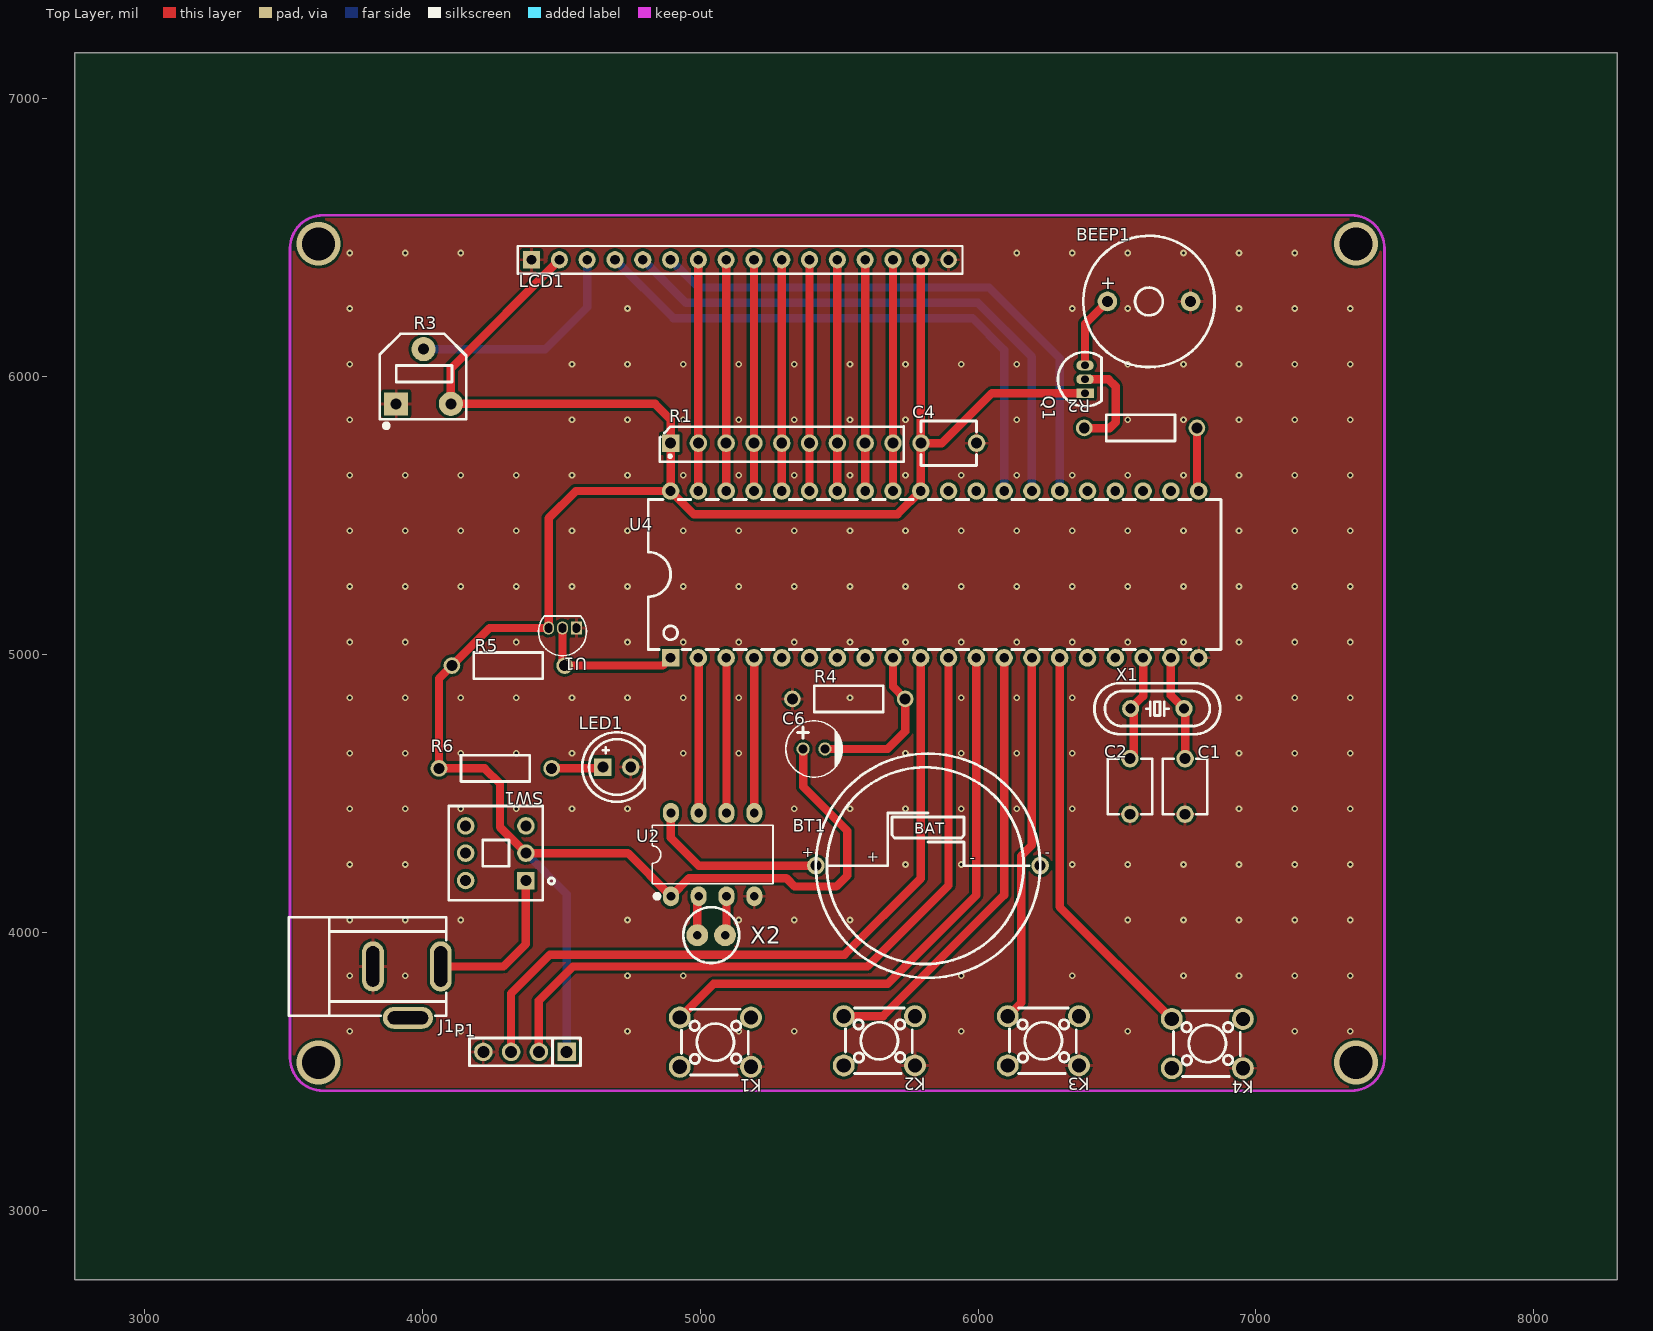
[diagram p0: Top Layer view]
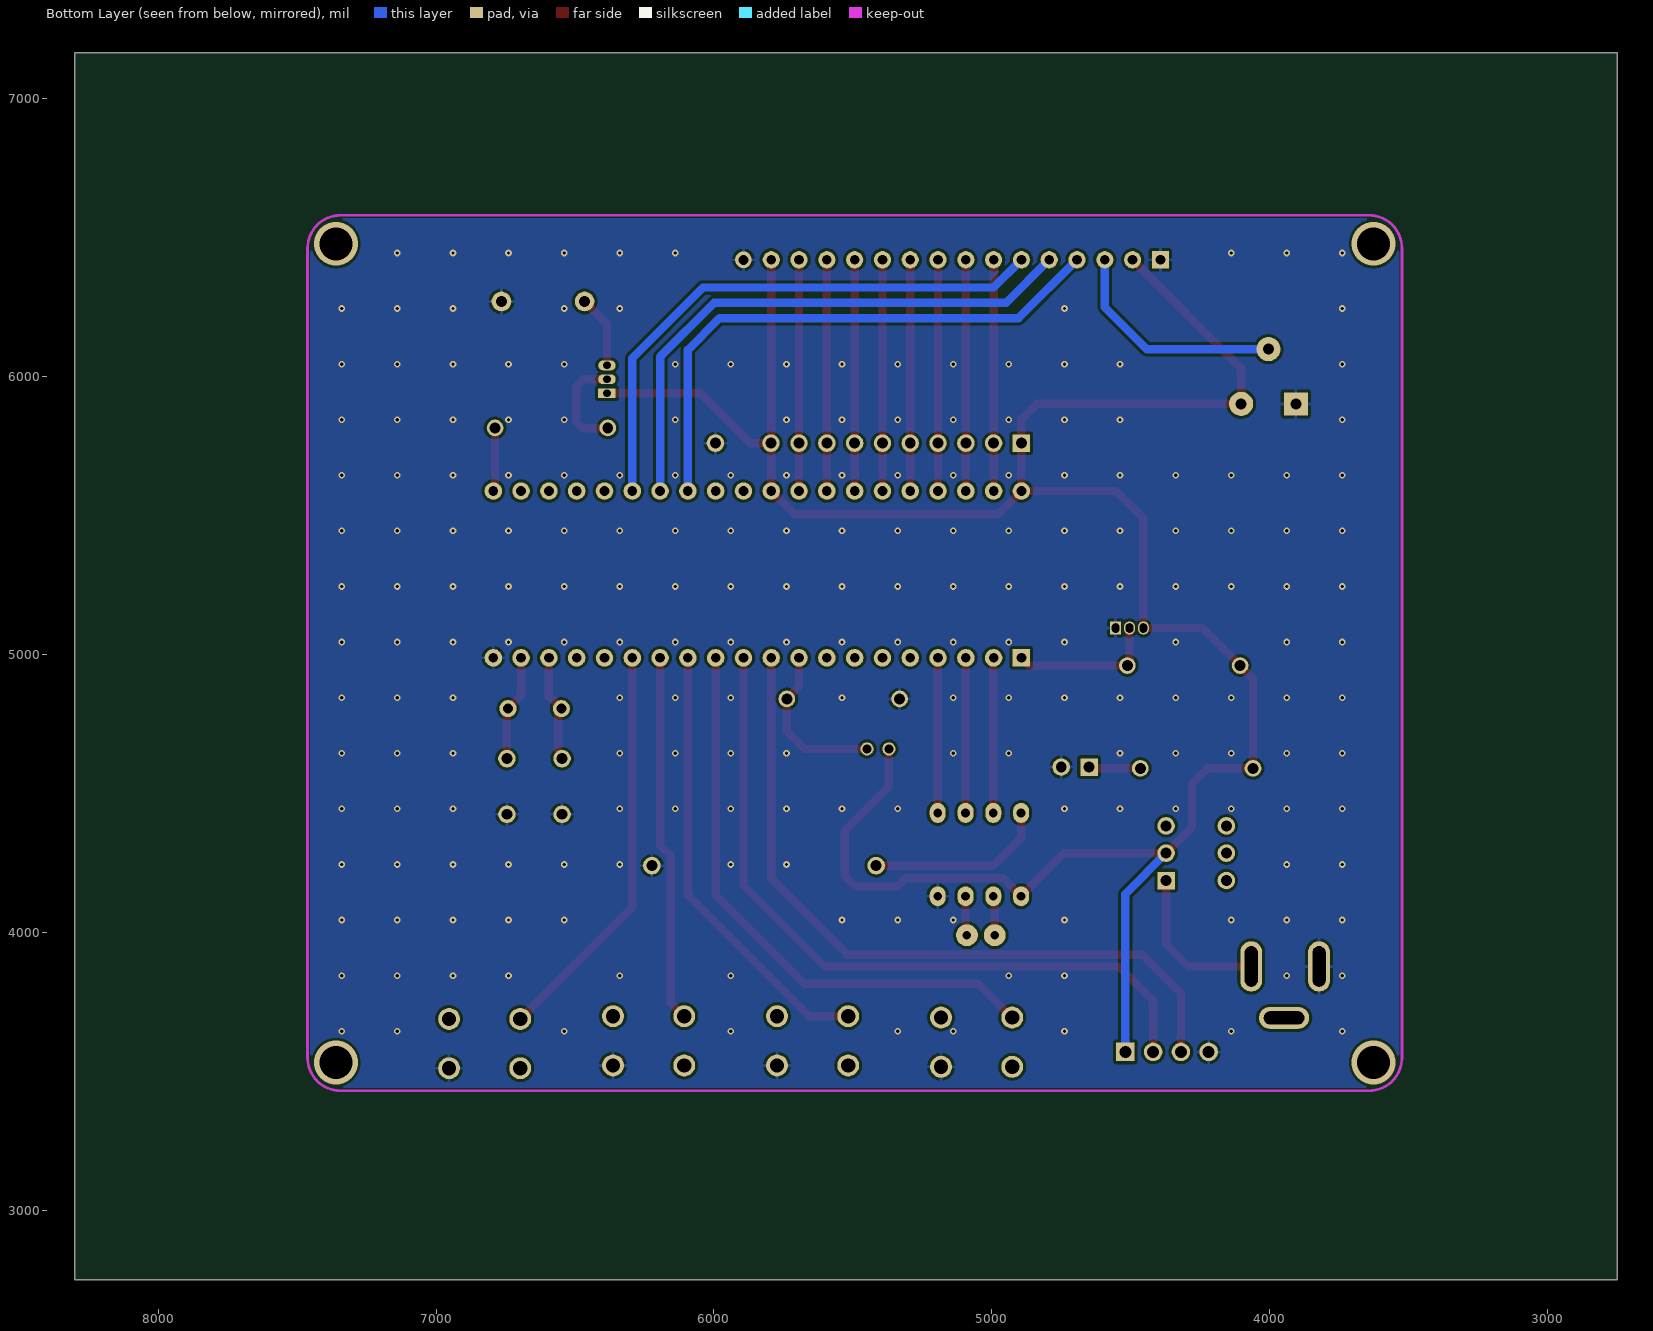
[diagram p1: Bottom Layer view, seen from below]
# Altium PCB MISC51236.pcbdoc
Units mil, origin at the board's own origin, x right, y up, seen from the top; angles counter-clockwise.
Board outline 5550 x 4415 mil, 2 copper layers (Top Layer, Bottom Layer), stack 62.206 mil thick; 27 components, 35 nets, 137 pads, 208 vias.

## Layer stack, top to bottom
Top Solder Mask Layer: solder mask 0.394, Dk 3.3
Top Layer: signal copper 1.379
Dielectric1: surface 59.449, FR4, Dk 4.5
Bottom Layer: signal copper 1.378
Bottom Solder Mask Layer: solder mask 0.394, Dk 3.3

## Board outline
8300,2750 2750,2750 2750,7165 8300,7165

## Design rules (kind name [scope] priority, off if disabled: settings)
BoardOutlineClearance copperThickness2oz_1 [All] p2 off: genericclearance=7.99 ignorepadtopadclearanceinfootprint=FALSE except(0: Arc-SplitContinuation Track-SplitContinuation SMDPad-SplitContinuation THPad-SplitContinuation Via-SplitContinuation Fill-SplitContinuation Region-SplitContinuation Poly-SplitContinuation Text-SplitContinuation Hole-SplitContinuation; 5.98: Arc-CutoutEdge SMDPad-CutoutEdge THPad-CutoutEdge Via-CutoutEdge Fill-CutoutEdge Region-CutoutEdge Text-CutoutEdge; 6.93: Hole-OutlineEdge Hole-CutoutEdge; 10: Poly-OutlineEdge Poly-CutoutEdge; 11.81: Arc-OutlineEdge Track-OutlineEdge SMDPad-OutlineEdge THPad-OutlineEdge Via-OutlineEdge Fill-OutlineEdge Region-OutlineEdge Text-OutlineEdge Track-CutoutEdge)
BoardOutlineClearance copperThickness1oz_1 [All] p4: genericclearance=4.02 ignorepadtopadclearanceinfootprint=FALSE except(0: Arc-SplitContinuation Track-SplitContinuation SMDPad-SplitContinuation THPad-SplitContinuation Via-SplitContinuation Fill-SplitContinuation Region-SplitContinuation Poly-SplitContinuation Text-SplitContinuation Hole-SplitContinuation; 6: SMDPad-CutoutEdge THPad-CutoutEdge Via-CutoutEdge Fill-CutoutEdge Region-CutoutEdge Text-CutoutEdge; 6.93: Hole-OutlineEdge Hole-CutoutEdge; 10: Poly-OutlineEdge Poly-CutoutEdge; 11.8: Arc-OutlineEdge Track-OutlineEdge SMDPad-OutlineEdge THPad-OutlineEdge Via-OutlineEdge Fill-OutlineEdge Region-OutlineEdge Text-OutlineEdge; 11.81: Arc-CutoutEdge Track-CutoutEdge)
Clearance copperThickness2oz [All] p1 off: gap=7.99 ignorepadtopadclearanceinfootprint=FALSE except(5.98: SMDPad-Track SMDPad-SMDPad THPad-Track SMDPad-THPad THPad-THPad Track-Via SMDPad-Via THPad-Via Via-Via Fill-Track Region-Track Fill-SMDPad Region-SMDPad Fill-THPad Region-THPad Fill-Via Region-Via Fill-Fill Fill-Region Region-Region Arc-Track Arc-SMDPad Arc-THPad Arc-Via Fill-Arc Region-Arc Arc-Arc Text-Track SMDPad-Text Text-THPad Text-Via Fill-Text Region-Text Arc-Text Text-Text; 6.93: Hole-Track Hole-SMDPad Hole-THPad Hole-Via Fill-Hole Region-Hole Hole-Arc Hole-Text; 10: Poly-Track Poly-SMDPad Poly-THPad Poly-Via Poly-Fill Poly-Region Poly-Poly Poly-Arc Poly-Text Poly-Hole)
Clearance copperThickness1oz [All] p3: gap=4.02 ignorepadtopadclearanceinfootprint=FALSE except(5.98: SMDPad-Track SMDPad-SMDPad THPad-Track SMDPad-THPad THPad-THPad Track-Via SMDPad-Via THPad-Via Via-Via Fill-Track Region-Track Fill-SMDPad Region-SMDPad Fill-THPad Region-THPad Fill-Via Region-Via Fill-Fill Fill-Region Region-Region; 6: Arc-Track Arc-SMDPad Arc-THPad Arc-Via Fill-Arc Region-Arc Arc-Arc Text-Track SMDPad-Text Text-THPad Text-Via Fill-Text Region-Text Arc-Text Text-Text; 6.93: Hole-Track Hole-SMDPad Hole-THPad Hole-Via Fill-Hole Region-Hole Hole-Arc Hole-Text; 10: Poly-Track Poly-SMDPad Poly-THPad Poly-Via Poly-Fill Poly-Region Poly-Poly Poly-Arc Poly-Text Poly-Hole)
DiffPairsRouting differentialPair [All] p1: maxlimit=6 minlimit=6 mostfreqgap=6 toplayer_minwidth=5 toplayer_prefwidth=10 toplayer_maxwidth=100 toplayer_mingap=6 toplayer_prefgap=6 toplayer_maxgap=6 bottomlayer_minwidth=5 bottomlayer_prefwidth=10 bottomlayer_maxwidth=100 bottomlayer_mingap=6 bottomlayer_prefgap=6 bottomlayer_maxgap=6 maxuncoupledlength=179724.41
HoleToHoleClearance otherClearance [All] p1: gap=11.81 allowstackedmicrovias=TRUE
Length netLength [All] p1: minlimit=0 maxlimit=0
MatchedLengths netLengthTolerance [All] p1: tolerance=1000
PasteMaskExpansion pasteMaskExpansion [All] p1: expansion=0
PlaneConnect innerPlane [All] p1: planeconnectstyle=Relief reliefexpansion=20 reliefentries=4 reliefconductorwidth=10 reliefairgap=10
PolygonConnect copperRegion [All] p1: connectstyle=Relief reliefconductorwidth=10 reliefentries=4 polygonreliefangle="90 Angle" airgapwidth=10 via.connectstyle=Relief via.reliefconductorwidth=10 via.reliefentries=4 via.polygonreliefangle="90 Angle" via.airgapwidth=10
RoutingVias viaSize [All] p1: holewidth=12.01 width=24.02 viastyle="Through Hole" minholewidth=11.81 minwidth=19.68 maxholewidth=248.03 maxwidth=393.7
SolderMaskExpansion solderMaskExpansion [IsVia] p1: expansion=-1000 istentingtop=TRUE
SolderMaskExpansion solderMaskExpansion [All] p2: expansion=2 istentingtop=FALSE
Width copperThickness2oz_2 [All] p1 off: maxlimit=100 minlimit=8 preferedwidth=10
Width copperThickness1oz_2 [All] p2: maxlimit=100 minlimit=5 preferedwidth=10

## Components (designator, comment, footprint, x,y, rotation, side; value= is the part's Value field where it differs from the comment)
BEEP1 "" BUZ-TH_BD12.0-P7.60-D0.6-FD 6615,6270 r0 top
BT1 "Battery" BAT-TH_CR2032 5820,4240 r0 top
C1 "30pF" CAP-TH_L5.0-W4.0-P5.00-D1.0 6745,4525 r90 top
C2 "30pF" CAP-TH_L5.0-W4.0-P5.00-D1.0 6546.5,4525 r90 top
C4 "0.1uF" CAP-TH_L5.0-W4.0-P5.00-D1.0 5895,5760 r0 top
C6 "10uF" CAP-TH_BD5.0-P2.00-D0.6-FD 5410,4660 r0 top
J1 "" DC-005_2.5 3940,3865 r180 top
K1 "" KEY-TH_4P-L6.0-W6.0-P4.50-LS6.50 5055,3605 r180 top
K2 "" KEY-TH_4P-L6.0-W6.0-P4.50-LS6.50 5645,3610 r180 top
K3 "" KEY-TH_4P-L6.0-W6.0-P4.50-LS6.50 6235,3610 r180 top
K4 "" KEY-TH_4P-L6.0-W6.0-P4.50-LS6.50 6825,3600 r180 top
LCD1 "1602" HDR-M-2.54_1X16 5143.88,6420 r0 top
LED1 "" LED-TH_5mm 4700.63,4595 r0 top
P1 "" HDR-TH_4P-P2.54-V-M 4370,3570 r180 top
Q1 "8550" S8550P_TO-92 6385,5990 r90 top
R1 "" SIP-9_L22.3-W3.2-P2.54_KA2284-SIP-9 5293.88,5760 r0 top
R2 "1K" Res_1/4W 6585,5815 r0 top
R3 "103" RES-ADJ-SMD_RM065-V1 4005,6000 r0 top
R4 "10K" Res_1/4W 5535,4840 r0 top
R5 "4.7K" Res_1/4W 4310,4960 r180 top
R6 "1K" Res_1/4W 4263.44,4590 r0 top
SW1 "SWT" SW-TH_6P-L8.5-W8.5-P2.50-LS5.5-BL-2 4265,4285 r90 top
U1 "DS18B20" TO-92-3_L4.5-W3.5-P1.27-L 4505,5095 r180 top
U2 "DS1302" DIP-8_L10.9-W6.4-P2.54-LS7.6-BL 5045,4280 r0 top
U4 "STC89C52RC-40I-PDIP40" DIP-40_L52.0-W13.7-P2.54-LS15.2-BL 5843.88,5287.97 r0 top
X1 "12M" HC-49S_L11.5-W4.7-P4.88 6645,4805 r0 top
X2 "32.768kHz" XTAL2 5090,3990 r180 top

## Footprints (in the part's own frame and the unit in brackets; to place one, negate y for a bottom-side part, rotate by r counter-clockwise, add the part's x,y. Pads: shape width x height; smd on the part's side, far side on the other; paste and mask are expansions set on the pad)
BAT-TH_CR2032 [mm]
  round 1.6 hole 1: 1(-10.25,0) 2(10.25,0)
  silkscreen extent -10.25,-10.25 10.25,10.25
BUZ-TH_BD12.0-P7.60-D0.6-FD [mm]
  round 1.8 hole 1: 1(-3.8,0) 2(3.8,0)
  silkscreen extent -6,-6 6,6
CAP-TH_BD5.0-P2.00-D0.6-FD [mm]
  round 1.201 hole 0.801: 1(-1,0) 2(1,0)
  silkscreen extent -2.58,-2.57 2.59,2.57
CAP-TH_L5.0-W4.0-P5.00-D1.0 [mm]
  round 1.6 hole 1: 1(-2.54,0) 2(2.54,0)
  silkscreen extent -2.54,-2.03 2.54,2.03
DC-005_2.5 [mm]
  oval 2x4.6 hole 1.2 slot 3.7 at 90 deg paste+0 mask+0.051: 1(-3.227,-0.318) 2(2.973,-0.318)
  oval 4.6x2 hole 1.2 slot 3.7 at 0 deg paste+0 mask+0.051: 3(-0.227,4.382)
  silkscreen extent -3.73,-4.82 10.67,4.18
DIP-8_L10.9-W6.4-P2.54-LS7.6-BL [mm]
  oval 1.462x1.828 hole 0.8: 1(-3.81,-3.81) 2(-1.27,-3.81) 3(1.27,-3.81) 4(3.81,-3.81) 5(3.81,3.81) 6(1.27,3.81) 7(-1.27,3.81) 8(-3.81,3.81)
  silkscreen extent -5.53,-4.01 5.53,2.67
DIP-40_L52.0-W13.7-P2.54-LS15.2-BL [mil]
  rect 63x63 hole 35: 1(-950,-300)
  round 63 hole 35: 2(-850,-300) 3(-750,-300) 4(-650,-300) 5(-550,-300) 6(-450,-300) 7(-350,-300) 8(-250,-300) 9(-150,-300) 10(-50,-300) 11(50,-300) 12(150,-300) 13(250,-300) 14(350,-300) 15(450,-300) 16(550,-300) 17(650,-300) 18(750,-300) 19(850,-300) 20(950,-300) 21(950,300) 22(850,300) 23(750,300) 24(650,300) 25(550,300) 26(450,300) 27(350,300) 28(250,300) 29(150,300) 30(50,300) 31(-50,300) 32(-150,300) 33(-250,300) 34(-350,300) 35(-450,300) 36(-550,300) 37(-650,300) 38(-750,300) 39(-850,300) 40(-950,300)
  silkscreen extent -1030,-270 1030,270
HC-49S_L11.5-W4.7-P4.88 [mm]
  round 1.56 hole 0.9: 1(-2.44,0) 2(2.44,0)
  silkscreen extent -5.75,-2.33 5.75,2.33
HDR-M-2.54_1X16 [mil]
  rect 62x62 hole 35: 1(-750,0)
  round 62 hole 35: 2(-650,0) 3(-550,0) 4(-450,0) 5(-350,0) 6(-250,0) 7(-150,0) 8(-50,0) 9(50,0) 10(150,0) 11(250,0) 12(350,0) 13(450,0) 14(550,0) 15(650,0)
  round 60 hole 36: 16(750,0)
  silkscreen extent -800,-50 800,50
HDR-TH_4P-P2.54-V-M [mm]
  rect 1.7x1.7 hole 1.1: 1(-3.81,0)
  round 1.7 hole 1.1: 2(-1.27,0) 3(1.27,0) 4(3.81,0)
  silkscreen extent -5.08,-1.27 5.08,1.27
KEY-TH_4P-L6.0-W6.0-P4.50-LS6.50 [mm]
  round 2 hole 1.3: 1(-3.25,2.25) 2(3.25,2.25) 3(-3.25,-2.25) 4(3.25,-2.25)
  silkscreen extent -3,-3 3.1,3
LED-TH_5mm [mm]
  rect 1.6x1.6 hole 1 paste+0 mask+0.051: 1(-1.27,0)
  round 1.6 hole 1 paste+0 mask+0.051: 2(1.27,0)
  silkscreen extent -3.17,-3.17 2.54,3.17
RES-ADJ-SMD_RM065-V1 [mm]
  rect 2.2x2.1 hole 1 paste+0 mask+0.05: 1(-2.5,-2.5)
  round 2.2 hole 1 paste+0 mask+0.05: 2(0,2.5) 3(2.5,-2.5)
  silkscreen extent -4,-4.7 3.9,3.9
Res_1/4W [mil]
  round 60 hole 39.37 paste+0 mask+2: 1(-202.76,0) 2(202.76,0)
  silkscreen extent -124,-47 124,47
S8550P_TO-92 [mm]
  rect 0.9x1.6 hole 0.7 paste+0 mask+0.051: 1(-1.27,0)
  oval 0.9x1.6 hole 0.7 paste+0 mask+0.051: 2(0,0) 3(1.27,0)
  silkscreen extent -2.48,-1.5 2.48,2.48
SIP-9_L22.3-W3.2-P2.54_KA2284-SIP-9 [mm]
  rect 1.6x1.6 hole 1: 1(-10.16,0)
  round 1.6 hole 1: 2(-7.62,0) 3(-5.08,0) 4(-2.54,0) 5(0,0) 6(2.54,0) 7(5.08,0) 8(7.62,0) 9(10.16,0)
  silkscreen extent -11.15,-1.69 11.15,1.52
SW-TH_6P-L8.5-W8.5-P2.50-LS5.5-BL-2 [mm]
  rect 1.6x1.6 hole 1: 1(-2.5,-2.75)
  round 1.6 hole 1: 2(0,-2.75) 3(2.5,-2.75) 4(2.5,2.75) 5(0,2.75) 6(-2.5,2.75)
  silkscreen extent -4.3,-5.36 4.3,4.3
TO-92-3_L4.5-W3.5-P1.27-L [mm]
  rect 1x1.2 hole 0.7 slot 0.85 at 90 deg: 1(-1.27,0)
  oval 1x1.2 hole 0.7 slot 0.85 at 90 deg: 2(0,0) 3(1.27,0)
  silkscreen extent -2.19,-1.1 2.19,2.52
XTAL2 [mm]
  round 2 hole 0.762: 1(0,0) 2(2.54,0)
  silkscreen extent -1.29,-2.55 3.83,2.55

## Via types
v1: diameter 24.02, hole 12, Top Layer to Bottom Layer, 204 vias
v2: diameter 157.48, hole 118.1, Top Layer to Bottom Layer, 4 vias

## Nets (pads, with @x,y where several pads share a name; then routed paths per layer and width w, separated by ;. In a path a pad name is that pad's centre, name@x,y a point inside that pad or via, vN(x,y) a via of type N, cw(c..) or ccw(c..) an arc to the next point about the centre after c; other vN are vias at no path point)
$2N34: J1.1 SW1.1 | length 568
  Top Layer w30: J1.1 4292.52,3877.51 4373.27,3958.27 SW1.1
$2N37: BEEP1.1 Q1.3 | length 263.3
  Top Layer w30: Q1.3 6385,6189.6 BEEP1.1
$2N47: U2.2 X2.2 | length 142.1
  Top Layer w30: X2.2 4990,4125 U2.2
$2N48: U2.3 X2.1 | length 142.1
  Top Layer w30: X2.1 5095,3995 U2.3
$2N51: BT1.1 U2.8 | length 652.9
  Top Layer w30: U2.8 4895,4340 4995,4240 BT1.1
$2N72: C6.2 R4.2 U4.9 | length 597.8
  Top Layer w30: C6.2 5675,4660 5737.76,4722.76 R4.2 5693.88,4883.88 U4.9
$2N199: LCD1.3 R3.2 | length 822.3
  Bottom Layer w30: R3.2 4443.43,6098.43 4593.88,6248.88 LCD1.3
$2N200: Q1.2 R2.1 | length 372.4
  Top Layer w30: R2.1 6383.45,5813.79 6473.79,5813.79 6495,5835 6495,5965 6470,5990 Q1.2
$2N202: LED1.1 R6.2 | length 186.5
  Top Layer w30: R6.2 4645.63,4590 LED1.1
BEEP: R2.2 U4.21 | length 229.6
  Top Layer w30: R2.2 6787.76,5594.09 U4.21
D0: LCD1.7 R1.2 U4.39 | length 832
  Top Layer w30: U4.39 R1.2 LCD1.7
D1: LCD1.8 R1.3 U4.38 | length 832
  Top Layer w30: U4.38 R1.3 LCD1.8
D2: LCD1.9 R1.4 U4.37 | length 832
  Top Layer w30: U4.37 R1.4 LCD1.9
D3: LCD1.10 R1.5 U4.36 | length 832
  Top Layer w30: U4.36 R1.5 LCD1.10
D4: LCD1.11 R1.6 U4.35 | length 832
  Top Layer w30: U4.35 R1.6 LCD1.11
D5: LCD1.12 R1.7 U4.34 | length 832
  Top Layer w30: U4.34 R1.7 LCD1.12
D6: LCD1.13 R1.8 U4.33 | length 832
  Top Layer w30: U4.33 R1.8 LCD1.13
D7: LCD1.14 R1.9 U4.32 | length 832
  Top Layer w30: U4.32 R1.9 LCD1.14
DQ: R5.1 U1.2 U4.1 | length 530.9
  Top Layer w30: U1.2 4505,4967.76 R5.1 4865.91,4960 U4.1
EN: LCD1.6 U4.26 | length 2024.7
  Bottom Layer w30: LCD1.6 4993.88,6320 6040,6320 6293.88,6066.12 U4.26
GND: BEEP1.2 BT1.2 C1.1 C2.1 C4.2 J1.2 K1.1 K2.1 K3.1 K4.1 LCD1.1 LCD1.16 LED1.2 P1.4 R3.1 R4.1 U1.1 U2.4 U4.20
  other v1: 3739.1,3644.49 4139.1,3644.49 4739.1,3644.49 5139.1,3644.49 5339.1,3644.49 5939.1,3644.49 6539.1,3644.49 7139.1,3644.49 7339.1,3644.49 3739.1,3844.49 3939.1,3844.49 4739.1,3844.49 4939.1,3844.49 5939.1,3844.49 6339.1,3844.49 6739.1,3844.49 6939.1,3844.49 7139.1,3844.49 7339.1,3844.49 3739.1,4044.49 3939.1,4044.49 4139.1,4044.49 4739.1,4044.49 5139.1,4044.49 5339.1,4044.49 5539.1,4044.49 6539.1,4044.49 6739.1,4044.49 6939.1,4044.49 7139.1,4044.49 7339.1,4044.49 3739.1,4244.49 3939.1,4244.49 5739.1,4244.49 5939.1,4244.49 6339.1,4244.49 6539.1,4244.49 6739.1,4244.49 6939.1,4244.49 7139.1,4244.49 7339.1,4244.49 3739.1,4444.49 3939.1,4444.49 4139.1,4444.49 4339.1,4444.49 4539.1,4444.49 4739.1,4444.49 5339.1,4444.49 5539.1,4444.49 5739.1,4444.49 5939.1,4444.49 6139.1,4444.49 6339.1,4444.49 6939.1,4444.49 7139.1,4444.49 7339.1,4444.49 3739.1,4644.49 3939.1,4644.49 4139.1,4644.49 4339.1,4644.49 4539.1,4644.49 4939.1,4644.49 5139.1,4644.49 5739.1,4644.49 5939.1,4644.49 6139.1,4644.49 6339.1,4644.49 6939.1,4644.49 7139.1,4644.49 7339.1,4644.49 3739.1,4844.49 3939.1,4844.49 4139.1,4844.49 4339.1,4844.49 4539.1,4844.49 4739.1,4844.49 4939.1,4844.49 5139.1,4844.49 5539.1,4844.49 5939.1,4844.49 6139.1,4844.49 6339.1,4844.49 6939.1,4844.49 7139.1,4844.49 7339.1,4844.49 3739.1,5044.49 3939.1,5044.49 4339.1,5044.49 4739.1,5044.49 4939.1,5044.49 5139.1,5044.49 5339.1,5044.49 5539.1,5044.49 5739.1,5044.49 5939.1,5044.49 6139.1,5044.49 6339.1,5044.49 6539.1,5044.49 6739.1,5044.49 6939.1,5044.49 7139.1,5044.49 7339.1,5044.49 3739.1,5244.49 3939.1,5244.49 4139.1,5244.49 4339.1,5244.49 4539.1,5244.49 4739.1,5244.49 4939.1,5244.49 5139.1,5244.49 5339.1,5244.49 5539.1,5244.49 5739.1,5244.49 5939.1,5244.49 6139.1,5244.49 6339.1,5244.49 6539.1,5244.49 6739.1,5244.49 6939.1,5244.49 7139.1,5244.49 7339.1,5244.49 3739.1,5444.49 3939.1,5444.49 4139.1,5444.49 4339.1,5444.49 4539.1,5444.49 4739.1,5444.49 4939.1,5444.49 5139.1,5444.49 5339.1,5444.49 5539.1,5444.49 5739.1,5444.49 5939.1,5444.49 6139.1,5444.49 6339.1,5444.49 6539.1,5444.49 6739.1,5444.49 6939.1,5444.49 7139.1,5444.49 7339.1,5444.49 3739.1,5644.49 3939.1,5644.49 4139.1,5644.49 4339.1,5644.49 4539.1,5644.49 4739.1,5644.49 4939.1,5644.49 5139.1,5644.49 5339.1,5644.49 5539.1,5644.49 5739.1,5644.49 5939.1,5644.49 6139.1,5644.49 6339.1,5644.49 6539.1,5644.49 6739.1,5644.49 6939.1,5644.49 7139.1,5644.49 7339.1,5644.49 3739.1,5844.49 4539.1,5844.49 4739.1,5844.49 4939.1,5844.49 5139.1,5844.49 5339.1,5844.49 5539.1,5844.49 5739.1,5844.49 6139.1,5844.49 6539.1,5844.49 6739.1,5844.49 6939.1,5844.49 7139.1,5844.49 7339.1,5844.49 3739.1,6044.49 4539.1,6044.49 4739.1,6044.49 4939.1,6044.49 5139.1,6044.49 5339.1,6044.49 5539.1,6044.49 5739.1,6044.49 5939.1,6044.49 6139.1,6044.49 6539.1,6044.49 6739.1,6044.49 6939.1,6044.49 7139.1,6044.49 7339.1,6044.49 3739.1,6244.49 4739.1,6244.49 6339.1,6244.49 6539.1,6244.49 6939.1,6244.49 7139.1,6244.49 7339.1,6244.49 3739.1,6444.49 3939.1,6444.49 4139.1,6444.49 6139.1,6444.49 6339.1,6444.49 6539.1,6444.49 6739.1,6444.49 6939.1,6444.49 7139.1,6444.49
IO: U2.6 U4.3 | length 558.4
  Top Layer w30: U4.3 5095,4986.85 U2.6
KEY1: K1.4 U4.12 | length 2103.3
  Top Layer w30: K1.4 5048.47,3815 5675,3815 5993.88,4133.88 U4.12
KEY2: K2.4 U4.13 | length 1611.2
  Top Layer w30: K2.4 5658.58,3698.58 6093.88,4133.88 U4.13
KEY3: K3.4 U4.14 | length 1325.4
  Top Layer w30: K3.4 6155,3746.53 6155,4275 6193.88,4313.88 U4.14
KEY4: K4.4 U4.15 | length 1466.4
  Top Layer w30: U4.15 6293.88,4091.75 K4.4
P3.0: P1.3 U4.10 | length 2649.4
  Top Layer w30: P1.3 4320,3780 4460,3920 5520,3920 5793.88,4193.88 U4.10
P3.1: P1.2 U4.11 | length 2649.4
  Top Layer w30: P1.2 4420,3755 4542.49,3877.49 5602.49,3877.49 5893.88,4168.88 U4.11
RS: LCD1.4 U4.28 | length 2042.3
  Bottom Layer w30: LCD1.4 4903.88,6210 5980,6210 6093.88,6096.12 U4.28
RST: U2.5 U4.4 | length 558.4
  Top Layer w30: U4.4 5195,4986.85 U2.5
RW: LCD1.5 U4.27 | length 2027.7
  Bottom Layer w30: LCD1.5 4948.88,6265 6000,6265 6193.88,6071.12 U4.27
SCLK: U2.7 U4.2 | length 558.4
  Top Layer w30: U4.2 4995,4986.85 U2.7
VCC: C4.1 C6.1 LCD1.2 LCD1.15 P1.1 Q1.1 R1.1 R3.3 R5.2 R6.1 SW1.2 U1.3 U2.1 U4.31 U4.40 | length 8988.9
  Top Layer w30: LCD1.2 4103.43,6029.55 R3.3 4838.43,5901.57 4893.88,5846.12 R1.1 U4.40 ; C6.1 5370.63,4524.37 5530,4365 5530,4205 5490,4165 5340,4165 5310,4195 4960,4195 U2.1 4740.01,4284.99 SW1.2 4280,4378.27 4280,4535 4225,4590 R6.1 4060.68,4913.44 R5.2 4242.24,5095 U1.3 4455,5490 4552.97,5587.97 U4.40 ; LCD1.15 U4.31 5710.91,5505 4976.85,5505 U4.40 ; C4.1 5870,5760 6050,5940 Q1.1
  Bottom Layer w30: SW1.2 4520,4138.27 P1.1
XTAL1: C1.2 U4.19 X1.2 | length 384.1
  Top Layer w30: U4.19 6693.88,4852.18 X1.2 6745,4801.06 C1.2
XTAL2: C2.2 U4.18 X1.1 | length 391.8
  Top Layer w30: C2.2 6560,4638.51 6560,4793.94 X1.1 6593.88,4849.94 U4.18
pads on no net: J1.3 K1.2 K1.3 K2.2 K2.3 K3.2 K3.3 K4.2 K4.3 SW1.3 SW1.4 SW1.5 SW1.6 U4.5 U4.6 U4.7 U4.8 U4.16 U4.17 U4.22 U4.23 U4.24 U4.25 U4.29 U4.30
copper on no net:
  other v2: 3627.36,3532.36 7359.65,3532.36 3627.36,6477.24 7359.65,6477.24

## Polygon pours and split planes (outlines as drawn)
GND on Bottom Layer (solid, remove dead copper, pour order 2): 3000,6915 3000,3000 8050,3000 8050,6915
GND on Top Layer (solid, remove dead copper, pour order 0): 3290,6780 3290,3240 7985,3240 7985,6780

## Keep-outs
Board Outline Layer:
  lines w10: 3525,3548.5 3525,6461.89 cw(c3643.11,6461.89) 3643.11,6580 7343.9,6580 cw(c7343.9,6461.89) 7462.01,6461.89 7462.01,3548.5 cw(c7343.9,3548.5) 7343.9,3430.39 3643.11,3430.39 cw(c3643.11,3548.5) 3525,3548.5